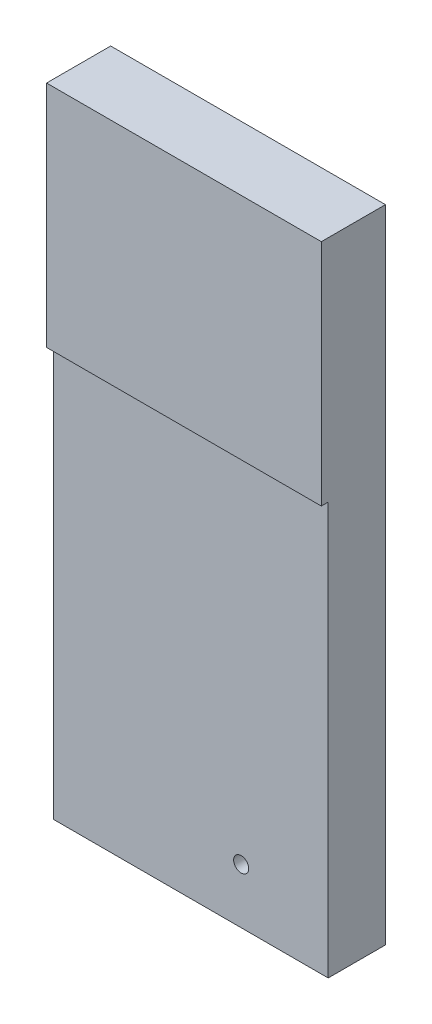
SolidWorks part; units mm, degrees
ref_plane "前视基准面" through (0, 0, 0) normal (0, 0, 1) x (1, 0, 0)
ref_plane "上视基准面" through (0, 0, 0) normal (0, 1, 0) x (1, 0, 0)
ref_plane "右视基准面" through (0, 0, 0) normal (1, 0, 0) x (0, 0, -1)
sketch "草图1" plane through (0, 0, 0) normal (0, 0, 1) x (1, 0, 0)
  line L1 (-30, -70) -> (30, -70)
  line L2 (-30, -70) -> (-30, 70)
  line L3 (-30, 70) -> (30, 70)
  line L4 (30, -70) -> (30, 70)
  line L5 (-30, -70) -> (30, 70) construction
  line L6 (-30, 70) -> (30, -70) construction
  point P0 (0, 0)
  dimension "D1" = 60
  dimension "D2" = 140
extrude "凸台-拉伸1" add sketch "草图1" along normal blind 14
sketch "草图2" plane through (0, 0, 14) normal (0, 0, 1) x (1, 0, 0)
  line L0 (30, -70) -> (30, 70) construction
  line L1 (-30, -70) -> (30, -70)
  line L2 (-30, -70) -> (-30, 20)
  line L3 (-30, 20) -> (30, 20)
  line L4 (30, -70) -> (30, 20)
  dimension "D1" = 90
extrude "切除-拉伸1" cut sketch "草图2" against normal blind 1.5
sketch "草图3" plane through (0, 0, 14) normal (0, 0, -1) x (-1, 0, 0)
  line L0 (-25, 70) -> (-25, 20)
  line L1 (-30, 70) -> (30, 70) construction
  line L2 (-30, -10) -> (30, -10)
  line L3 (35, 20) -> (35, 70)
  line L4 (35, 70) -> (-25, 70)
  line L5 (35, 20) -> (30, 20)
  line L7 (-30, -70) -> (-30, 70) construction
  line L8 (30, 70) -> (30, -70) construction
  line L9 (30, 20) -> (30, -10)
  line L10 (-25, 20) -> (-30, 20)
  line L11 (-30, 20) -> (-30, 70) construction
  line L12 (-30, 20) -> (-30, -10)
  dimension "D4" = 80
  dimension "D1" = 5
  dimension "D3" = 60
  dimension "D5" = 30
extrude "切除-拉伸2" [suppressed] cut sketch "草图3" along normal blind 1.5
hole_wizard "M4 螺纹孔1" positions "草图5" profile "草图4" tap size "M4" standard "GB" end condition through all
sketch "草图5" plane through (0, 0, 0) normal (0, 0, -1) x (-1, 0, 0)
  line L0 (30, -70) -> (-30, -70) construction
  line L1 (-30, -70) -> (-30, 70) construction
  point P1 (-11, -58)
  dimension "D1" = 12
  dimension "D2" = 19
sketch "草图4" plane through (11, -58, 0) normal (1, 0, 0) x (0, 1, 0)
  line L0 (0, 0) -> (0, 14)
  line L1 (0, 14) -> (1.65, 14)
  line L2 (1.65, 14) -> (1.65, 0)
  line L5 (1.65, 0) -> (0, 0)
  line L11 (0, -6.35) -> (0, 107.95) construction
  dimension "通孔螺纹孔钻头直径" = 3.3
  dimension "通孔螺纹孔钻头深度" = 14
cosmetic thread "孔螺蚊线1" parameters "D2"=4
sketch "草图6" plane through (0, 0, 0) normal (0, 0, -1) x (-1, 0, 0)
  line L0 (30, -24) -> (22, -24)
  line L1 (30, 70) -> (30, -70) construction
  line L2 (22, -24) -> (22, -42)
  line L3 (22, -42) -> (30, -42)
  line L4 (30, -42) -> (30, -24)
  line L5 (30, -70) -> (-30, -70) construction
  dimension "D1" = 18
  dimension "D2" = 28
  dimension "D3" = 8
extrude "切除-拉伸3" [suppressed] cut sketch "草图6" against normal up to next
fillet "圆角1" [suppressed] radius 2
